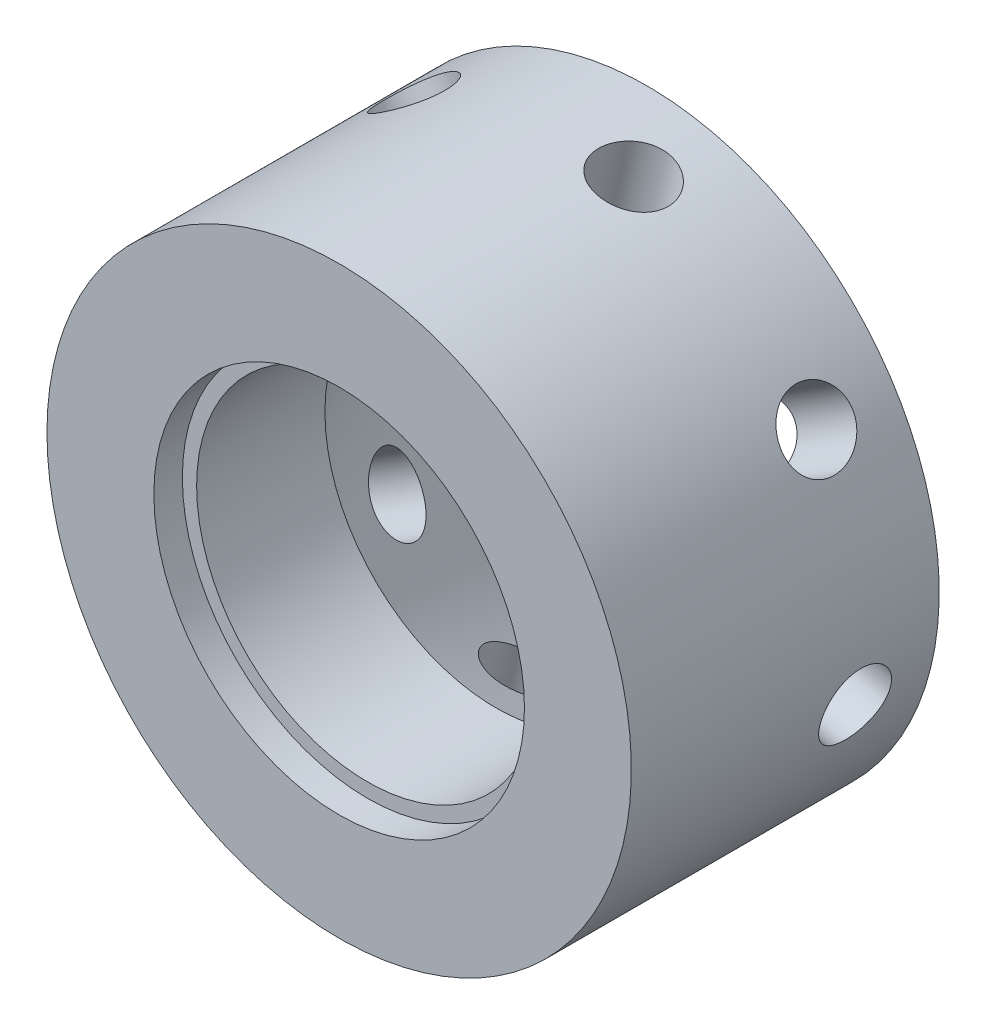
from build123d import *

# Parameters (mm, degrees)
SKETCH1_W                       = 102.5
SKETCH1_H                       = 108
F_25_0_25_DIAMETER_HOLE1_REACH  = 260.996
F_25_0_25_DIAMETER_HOLE1_BORE_R = 12.5
F_25_0_25_DIAMETER_HOLE2_REACH  = 253.343
F_25_0_25_DIAMETER_HOLE2_BORE_R = 12.5
F_25_0_25_DIAMETER_HOLE3_REACH  = 260.996
F_25_0_25_DIAMETER_HOLE3_BORE_R = 12.5
F_25_0_25_DIAMETER_HOLE4_REACH  = 253.343
F_25_0_25_DIAMETER_HOLE4_BORE_R = 12.5
F_25_0_25_DIAMETER_HOLE5_D      = 25
F_25_0_25_DIAMETER_HOLE5_DEPTH  = 243.959427947
F_25_0_25_DIAMETER_HOLE6_D      = 25
F_25_0_25_DIAMETER_HOLE6_DEPTH  = 224.906936905
F_25_0_25_DIAMETER_HOLE7_D      = 25
F_25_0_25_DIAMETER_HOLE7_DEPTH  = 243.959427947
F_25_0_25_DIAMETER_HOLE8_D      = 25
F_25_0_25_DIAMETER_HOLE8_DEPTH  = 224.906936905


with BuildPart() as part:
    # Sketch1 → Revolve1 (revolve)
    with BuildSketch(Plane.XZ.offset(-234.743963655), mode=Mode.PRIVATE) as revolve1_sk:
        with Locations((572.480642584, -1098.692981355)):
            Rectangle(SKETCH1_W, SKETCH1_H)
    revolve(revolve1_sk.sketch.rotate(Axis((521.230642584, 234.743963655, -1044.692981355), (0, 0, -1)), 180), axis=Axis((521.230642584, 234.743963655, -1044.692981355), (0, 0, -1)))

    # Sketch2 → Cut-Revolve1 (revolve, cut)
    with BuildSketch(Plane(origin=(0, 234.743963655, 0), x_dir=(1, 0, 0), z_dir=(0, 1, 0))):
        Polygon((606.230642584, 1152.692981355), (521.230642584, 1152.692981355), (521.230642584, 1044.692981355), (586.230642584, 1044.692981355), (586.230642584, 1054.692981355), (581.230642584, 1054.692981355), (581.230642584, 1099.692981355), align=None)
    revolve(axis=Axis((521.230642584, 234.743963655, -1152.692981355), (0, 0, 1)), mode=Mode.SUBTRACT)

    # Ø25.0 (25) diameter hole1 bore (on position points) → Ø25.0 (25) diameter hole1 (cut, up to next)
    with BuildSketch(Plane(origin=(434.675867434, 179.839310858, -1125.692981355), x_dir=(0.535655149238, -0.844436830731, 0), z_dir=(-0.844436830731, -0.535655149238, 0)), mode=Mode.PRIVATE) as f_25_0_25_diameter_hole1_sk1:
        with Locations((1e-09, 0)):
            Circle(F_25_0_25_DIAMETER_HOLE1_BORE_R)
    f_25_0_25_diameter_hole1_tool1 = extrude(f_25_0_25_diameter_hole1_sk1.sketch, amount=-F_25_0_25_DIAMETER_HOLE1_REACH, mode=Mode.PRIVATE) & part.part
    add(f_25_0_25_diameter_hole1_tool1.solids().sort_by_distance((434.675867, 179.839311, -1125.692981))[0], mode=Mode.SUBTRACT)

    # Ø25.0 (25) diameter hole2 bore (on position points) → Ø25.0 (25) diameter hole2 (cut, up to next)
    with BuildSketch(Plane(origin=(421.20372182, 257.123979796, -1125.692981355), x_dir=(-0.21834162089, -0.975872397697, 0), z_dir=(-0.975872397697, 0.21834162089, 0)), mode=Mode.PRIVATE) as f_25_0_25_diameter_hole2_sk1:
        Circle(F_25_0_25_DIAMETER_HOLE2_BORE_R)
    f_25_0_25_diameter_hole2_tool1 = extrude(f_25_0_25_diameter_hole2_sk1.sketch, amount=-F_25_0_25_DIAMETER_HOLE2_REACH, mode=Mode.PRIVATE) & part.part
    add(f_25_0_25_diameter_hole2_tool1.solids().sort_by_distance((421.203722, 257.12398, -1125.692981))[0], mode=Mode.SUBTRACT)

    # Ø25.0 (25) diameter hole3 bore (on position points) → Ø25.0 (25) diameter hole3 (cut, up to next)
    with BuildSketch(Plane(origin=(466.325989788, 321.298738804, -1125.692981355), x_dir=(0.844436830731, 0.535655149238, 0), z_dir=(-0.535655149238, 0.844436830731, 0)), mode=Mode.PRIVATE) as f_25_0_25_diameter_hole3_sk1:
        Circle(F_25_0_25_DIAMETER_HOLE3_BORE_R)
    f_25_0_25_diameter_hole3_tool1 = extrude(f_25_0_25_diameter_hole3_sk1.sketch, amount=-F_25_0_25_DIAMETER_HOLE3_REACH, mode=Mode.PRIVATE) & part.part
    add(f_25_0_25_diameter_hole3_tool1.solids().sort_by_distance((466.32599, 321.298739, -1125.692981))[0], mode=Mode.SUBTRACT)

    # Ø25.0 (25) diameter hole4 bore (on position points) → Ø25.0 (25) diameter hole4 (cut, up to next)
    with BuildSketch(Plane(origin=(543.610658726, 334.770884418, -1125.692981355), x_dir=(0.975872397697, -0.21834162089, 0), z_dir=(0.21834162089, 0.975872397697, 0)), mode=Mode.PRIVATE) as f_25_0_25_diameter_hole4_sk1:
        Circle(F_25_0_25_DIAMETER_HOLE4_BORE_R)
    f_25_0_25_diameter_hole4_tool1 = extrude(f_25_0_25_diameter_hole4_sk1.sketch, amount=-F_25_0_25_DIAMETER_HOLE4_REACH, mode=Mode.PRIVATE) & part.part
    add(f_25_0_25_diameter_hole4_tool1.solids().sort_by_distance((543.610659, 334.770884, -1125.692981))[0], mode=Mode.SUBTRACT)

    # Ø25.0 (25) diameter hole5
    with Locations(Plane(origin=(607.785417734, 289.648616451, -1125.692981355), x_dir=(-0.535655149238, 0.844436830731, 0), z_dir=(0.844436830731, 0.535655149238, 0))):
        with Locations((0, 0)):
            Hole(F_25_0_25_DIAMETER_HOLE5_D / 2, depth=F_25_0_25_DIAMETER_HOLE5_DEPTH)

    # Ø25.0 (25) diameter hole6
    with Locations(Plane(origin=(621.257563348, 212.363947513, -1125.692981355), x_dir=(0.21834162089, 0.975872397697, 0), z_dir=(0.975872397697, -0.21834162089, 0))):
        with Locations((0, 0)):
            Hole(F_25_0_25_DIAMETER_HOLE6_D / 2, depth=F_25_0_25_DIAMETER_HOLE6_DEPTH)

    # Ø25.0 (25) diameter hole7
    with Locations(Plane(origin=(576.135295381, 148.189188505, -1125.692981355), x_dir=(-0.844436830731, -0.535655149238, 0), z_dir=(0.535655149238, -0.844436830731, 0))):
        with Locations((0, 0)):
            Hole(F_25_0_25_DIAMETER_HOLE7_D / 2, depth=F_25_0_25_DIAMETER_HOLE7_DEPTH)

    # Ø25.0 (25) diameter hole8
    with Locations(Plane(origin=(498.850626443, 134.717042891, -1125.692981355), x_dir=(-0.975872397697, 0.21834162089, 0), z_dir=(-0.21834162089, -0.975872397697, 0))):
        with Locations((0, 0)):
            Hole(F_25_0_25_DIAMETER_HOLE8_D / 2, depth=F_25_0_25_DIAMETER_HOLE8_DEPTH)


solid = part.part
